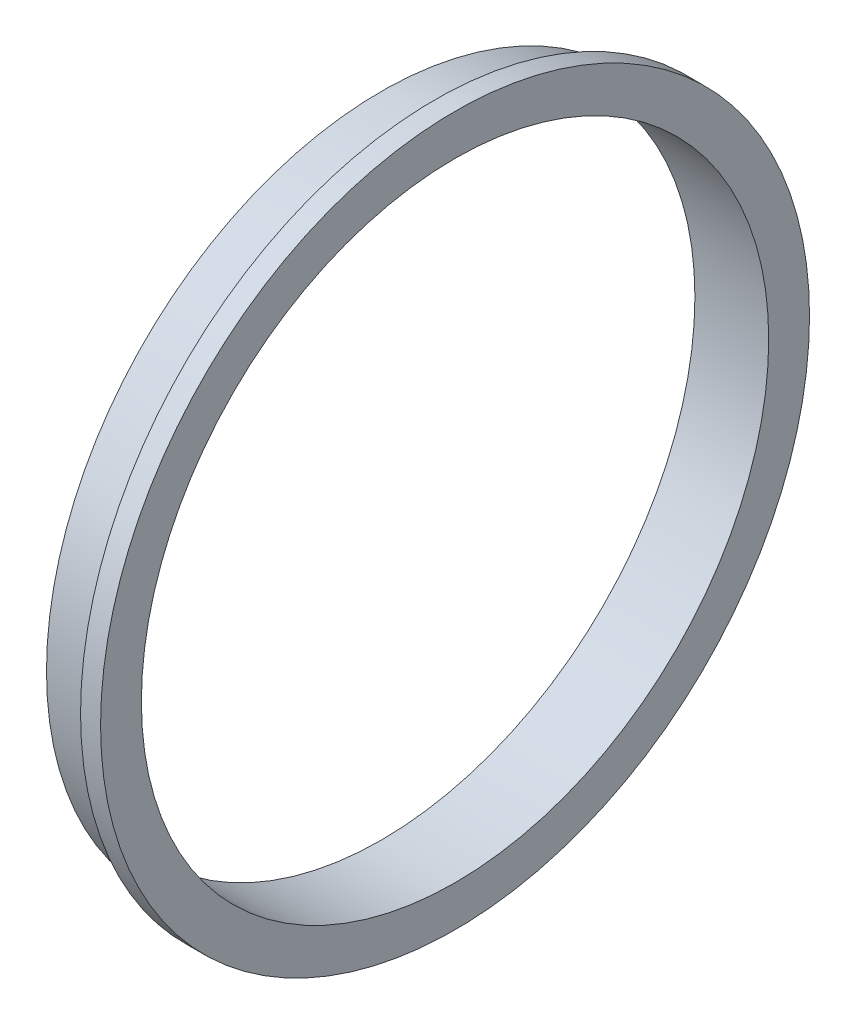
SolidWorks part; units mm, degrees
material "普通碳钢"
ref_plane "前视" through (0, 0, 0) normal (0, 0, 1) x (1, 0, 0)
ref_plane "上视" through (0, 0, 0) normal (0, 1, 0) x (1, 0, 0)
ref_plane "右视" through (0, 0, 0) normal (1, 0, 0) x (0, 0, -1)
sketch "草图1" plane through (0, 0, 0) normal (0, 0, 1) x (1, 0, 0)
  line L0 (-185.1316, 0) -> (218.2895, 0) construction
  line L1 (0, 138.3882) -> (0, -124.5724) construction
  line L2 (0, 297.5) -> (70, 297.5)
  line L3 (70, 297.5) -> (70, 336.2)
  line L4 (70, 336.2) -> (51, 336.2)
  line L5 (51, 336.2) -> (51, 317.5)
  line L6 (51, 317.5) -> (0, 317.5)
  line L7 (0, 317.5) -> (0, 297.5)
  dimension "D1" = 70
  dimension "D2" = 38.7
  dimension "D3" = 19
  dimension "D4" = 20
  dimension "D5" = 297.5
revolve "旋转1" add sketch "草图1" angle 360 about L0
